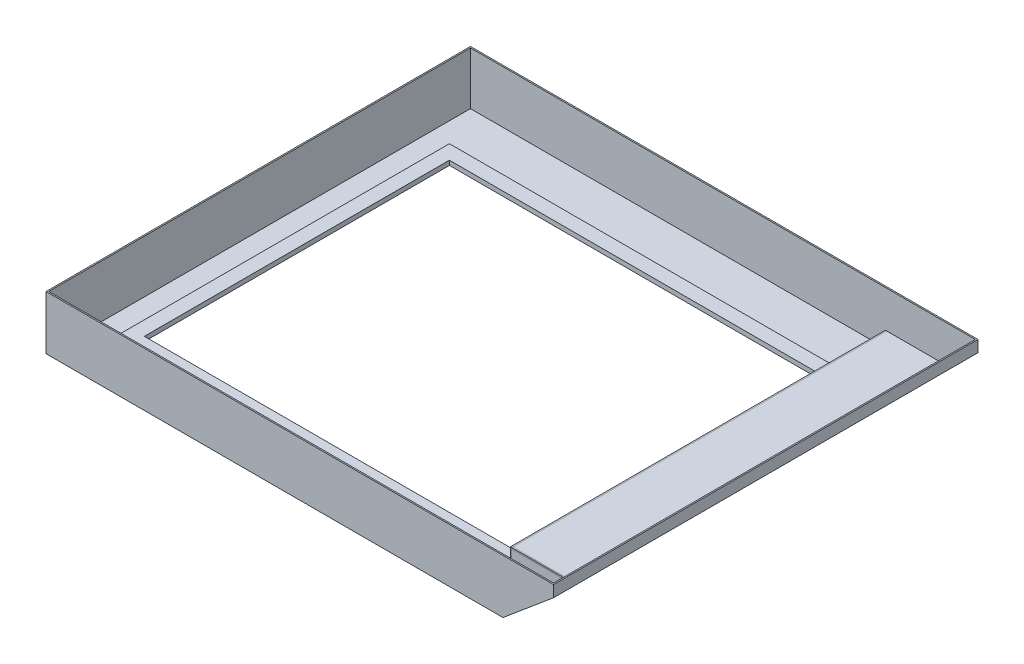
from build123d import *

# Parameters (mm, degrees)
EXTRUDE_1_DEPTH      = 654
SKETCH_8_W           = 110.00435438
SKETCH_8_H           = 134.15256119
CUT_EXTRUDE_2_DEPTH  = 799
SHELL_1_T            = -2
SKETCH_3_W           = 75
SKETCH_3_H           = 574
CUT_EXTRUDE_1_DEPTH  = 654
SKETCH_5_W           = 2
SKETCH_5_H           = 578
EXTRUDE_2_DEPTH      = 60
EXTRUDE_3_DEPTH      = 289
EXTRUDE_3_DEPTH_BACK = 289
EXTRUDE_5_DEPTH      = 2
EXTRUDE_6_DEPTH      = 2
SKETCH_11_W          = 585
SKETCH_11_H          = 470
CUT_EXTRUDE_3_DEPTH  = 2
SKETCH_12_W          = 589
SKETCH_12_H          = 474
SKETCH_12_W_2        = 585
SKETCH_12_H_2        = 470
EXTRUDE_7_DEPTH      = 5
SKETCH_15_W          = 629
SKETCH_15_H          = 514
SKETCH_15_W_2        = 585
SKETCH_15_H_2        = 470
EXTRUDE_8_DEPTH      = 2


with BuildPart() as part:
    # 草图2 → 凸台-拉伸1 (new body)
    with BuildSketch(Plane.XY):
        Polygon((0, 0), (0, 83), (784, 83), (784, 67), (704.152509296, 0), align=None)
    extrude(amount=EXTRUDE_1_DEPTH)

    # 草图8 → 切除-拉伸2 (cut)
    with BuildSketch(Plane.XY.offset(654)):
        with Locations((837.00217719, 67.076280595)):
            Rectangle(SKETCH_8_W, SKETCH_8_H)
    extrude(amount=-CUT_EXTRUDE_2_DEPTH, mode=Mode.SUBTRACT)

    # 抽壳1
    shell_1_openings = [part.faces().sort_by_distance(p)[0] for p in [
        (391, 83, 327),
    ]]
    offset(amount=SHELL_1_T, openings=shell_1_openings, kind=Kind.INTERSECTION)

    # 草图3 → 切除-拉伸1 (cut)
    with BuildSketch(Plane(origin=(290.938854629, -346.727425229, 0), x_dir=(0.7660444431189772, 0.6427876096865405, 0), z_dir=(0.6427876096865404, -0.7660444431189772, 0))):
        with Locations((590.223457765, 327)):
            Rectangle(SKETCH_3_W, SKETCH_3_H)
    extrude(amount=-CUT_EXTRUDE_1_DEPTH, mode=Mode.SUBTRACT)

    # 草图5 → 凸台-拉伸2 (add)
    with BuildSketch(Plane(origin=(0, 2, 0), x_dir=(1, 0, 0), z_dir=(0, 1, 0))):
        with Locations((678.424568828, -327)):
            Rectangle(SKETCH_5_W, SKETCH_5_H)
    extrude(amount=EXTRUDE_2_DEPTH)

    # 草图11 → 切除-拉伸3 (cut)
    with BuildSketch(Plane.XZ):
        with Locations((352.076254648, 327)):
            Rectangle(SKETCH_11_W, SKETCH_11_H)
    extrude(amount=-CUT_EXTRUDE_3_DEPTH, mode=Mode.SUBTRACT)

    # 草图12 → 凸台-拉伸7 (add)
    with BuildSketch(Plane(origin=(0, 2, 0), x_dir=(1, 0, 0), z_dir=(0, 1, 0))):
        with Locations((352.076254648, -327)):
            Rectangle(SKETCH_12_W, SKETCH_12_H)
        with Locations((352.076254648, -327)):
            Rectangle(SKETCH_12_W_2, SKETCH_12_H_2, mode=Mode.SUBTRACT)
    extrude(amount=EXTRUDE_7_DEPTH)

    # 草图15 → 凸台-拉伸8 (add)
    with BuildSketch(Plane(origin=(0, 7, 0), x_dir=(1, 0, 0), z_dir=(0, 1, 0))):
        with Locations((352.076254648, -327)):
            Rectangle(SKETCH_15_W, SKETCH_15_H)
        with Locations((352.076254648, -327)):
            Rectangle(SKETCH_15_W_2, SKETCH_15_H_2, mode=Mode.SUBTRACT)
    extrude(amount=-EXTRUDE_8_DEPTH)


with BuildPart() as body_2:
    # 草图6 → 凸台-拉伸3 (new, two sides: drawn at the far end of the back side and taken through both)
    with BuildSketch(Plane.XY.offset(327).offset(-EXTRUDE_3_DEPTH_BACK)):
        Polygon((679.424568828, 62), (774.929784383, 62), (772.546277198, 60), (681.424568828, 60), (681.424568828, 4), (702.696628359, 4), (746.250437533, 40.545985214), (747.536012752, 39.013896328), (703.424568828, 2), (679.424568828, 2), align=None)
    extrude(amount=EXTRUDE_3_DEPTH + EXTRUDE_3_DEPTH_BACK)


with BuildPart() as body_3:
    # 草图9 → 凸台-拉伸5 (new body)
    with BuildSketch(Plane.XY.offset(616)):
        Polygon((679.424568828, 62), (679.424568828, 2), (703.424568828, 2), (774.929784383, 62), align=None)
    extrude(amount=-EXTRUDE_5_DEPTH)


with BuildPart() as body_4:
    # 草图10 → 凸台-拉伸6 (new body)
    with BuildSketch(Plane(origin=(0, 0, 38), x_dir=(-1, 0, 0), z_dir=(0, 0, -1))):
        Polygon((-679.424568828, 2), (-679.424568828, 62), (-774.929784383, 62), (-703.424568828, 2), align=None)
    extrude(amount=-EXTRUDE_6_DEPTH)


solid = Compound([part.part, body_2.part, body_3.part, body_4.part])
